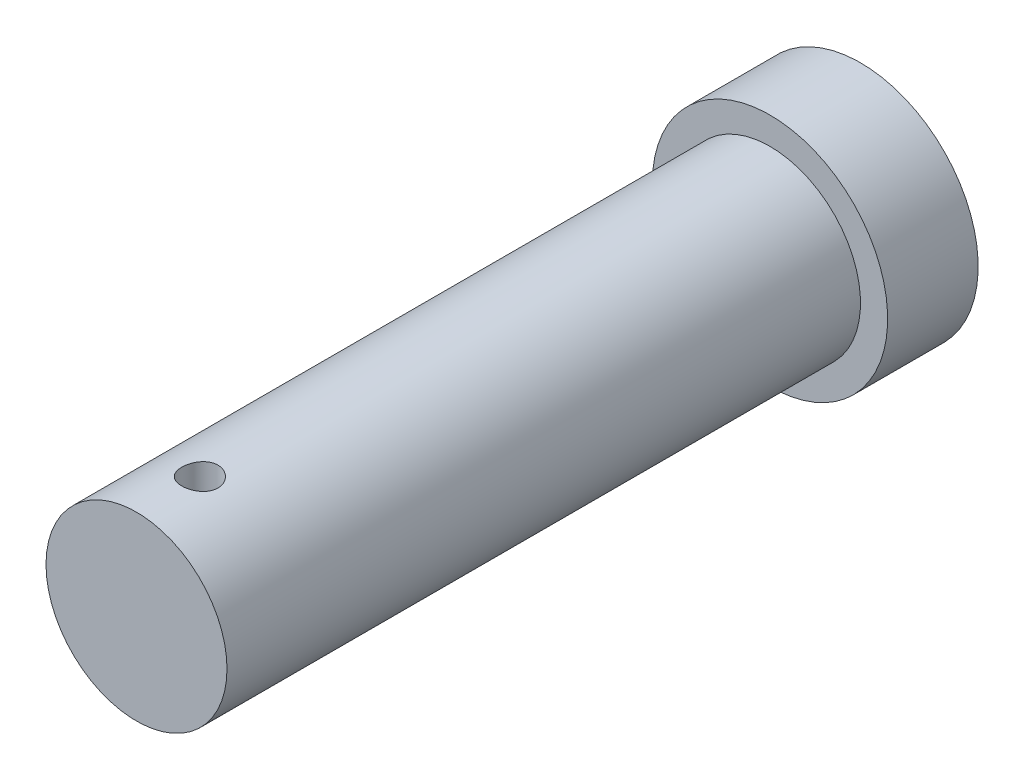
SolidWorks part; units mm, degrees
material "06Cr19Ni10"
ref_plane "Front" through (0, 0, 0) normal (0, 0, 1) x (1, 0, 0)
ref_plane "Top" through (0, 0, 0) normal (0, 1, 0) x (1, 0, 0)
ref_plane "Right" through (0, 0, 0) normal (1, 0, 0) x (0, 0, -1)
sketch "Sketch1" plane through (0, 0, 0) normal (0, 0, 1) x (1, 0, 0)
  circle A0 centre (0, 0) radius 10
  dimension "D1" = 20
extrude "Boss-Extrude1" add sketch "Sketch1" along normal blind 70
sketch "Sketch2" plane through (0, 0, 0) normal (0, 0, -1) x (-1, 0, 0)
  circle A0 centre (0, 0) radius 13
  dimension "D1" = 26
extrude "Boss-Extrude2" add sketch "Sketch2" along normal blind 10
sketch "Sketch3" plane through (0, 0, 0) normal (0, 1, 0) x (1, 0, 0)
  line L0 (-10, -70) -> (10, -70) construction
  circle A0 centre (0, -63) radius 2
  dimension "D1" = 4
  dimension "D2" = 7
extrude "Cut-Extrude1" cut sketch "Sketch3" against normal through all both and the other way through all
equation "\"零件重量\"= IIF ( \"SW-质量\" > 100 , int ( \"SW-质量\" ) , \"SW-质量\" )"
